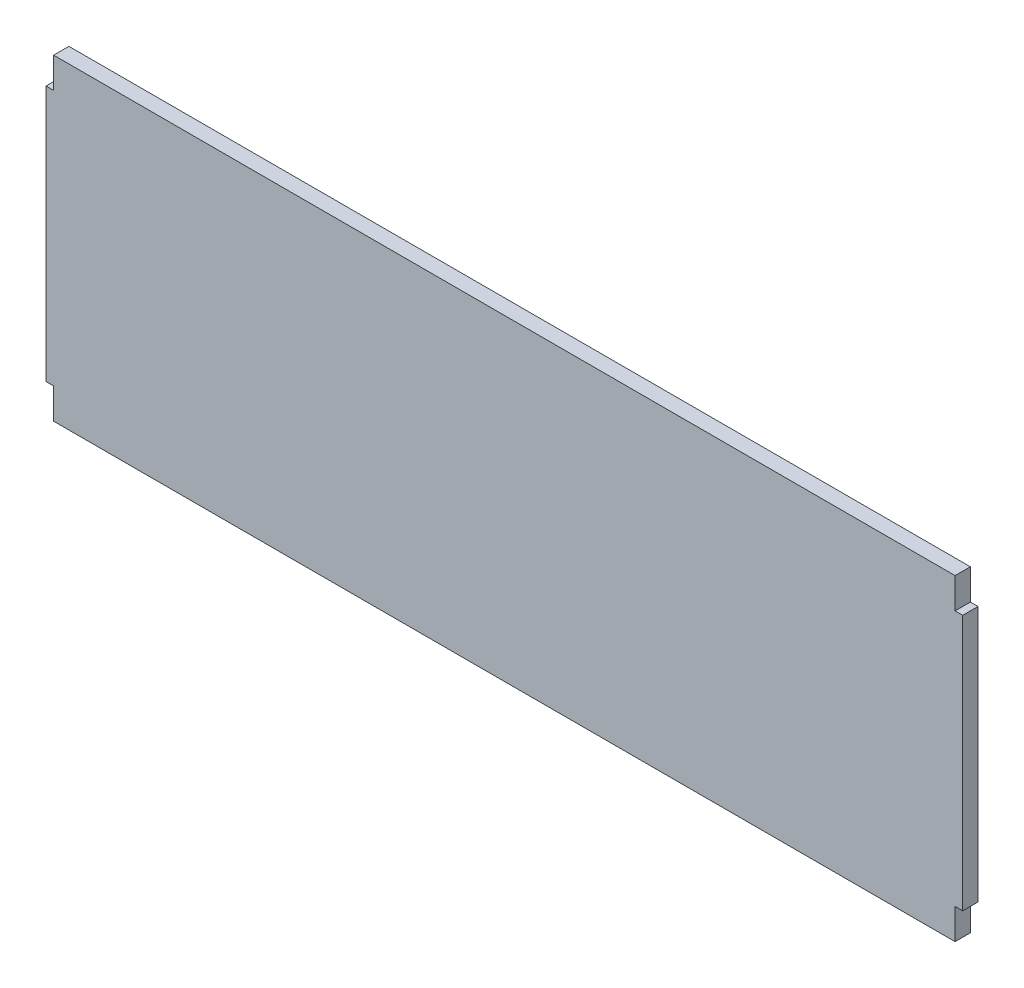
SolidWorks part; units mm, degrees
ref_plane "Front Plane" through (0, 0, 0) normal (0, 0, 1) x (1, 0, 0)
ref_plane "Top Plane" through (0, 0, 0) normal (0, 1, 0) x (1, 0, 0)
ref_plane "Right Plane" through (0, 0, 0) normal (1, 0, 0) x (0, 0, -1)
sketch "Sketch1" plane through (0, 0, 0) normal (0, 0, 1) x (1, 0, 0)
  line L1 (0, 0) -> (1200, 0)
  line L2 (0, 0) -> (0, 415)
  line L3 (0, 415) -> (1200, 415)
  line L4 (1200, 0) -> (1200, 415)
extrude "Boss-Extrude1" add sketch "Sketch1" along normal blind 20
sketch "Sketch2" plane through (0, 0, 20) normal (0, 0, 1) x (1, 0, 0)
  line L0 (1200, 415) -> (0, 415) construction
  line L1 (0, 415) -> (10, 415)
  line L2 (0, 415) -> (0, 375)
  line L3 (0, 375) -> (10, 375)
  line L4 (10, 415) -> (10, 375)
  line L5 (1190, 415) -> (1200, 415)
  line L6 (1190, 415) -> (1190, 375)
  line L7 (1190, 375) -> (1200, 375)
  line L8 (1200, 415) -> (1200, 375)
  line L9 (1200, 0) -> (1200, 415) construction
  line L11 (1200, 0) -> (1190, 0)
  line L12 (1200, 0) -> (1200, 40)
  line L13 (1200, 40) -> (1190, 40)
  line L14 (1190, 0) -> (1190, 40)
  line L15 (0, 0) -> (10, 0)
  line L16 (0, 0) -> (0, 40)
  line L17 (0, 40) -> (10, 40)
  line L18 (10, 0) -> (10, 40)
extrude "Cut-Extrude1" cut sketch "Sketch2" against normal blind 280
